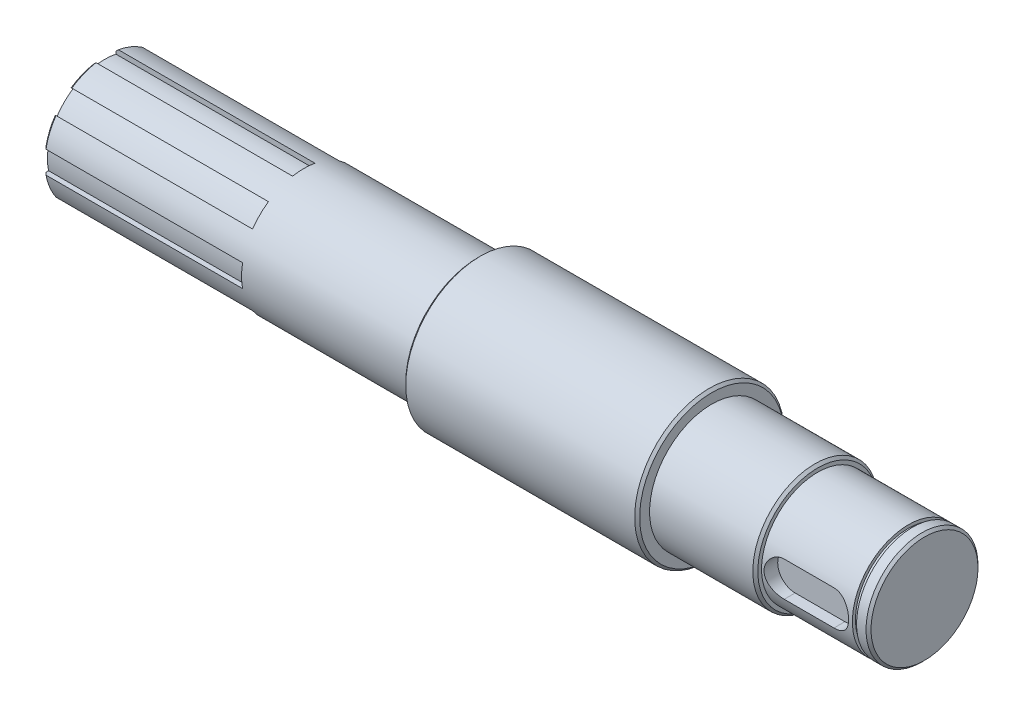
SolidWorks part; units mm, degrees
ref_plane "前视基准面" through (0, 0, 0) normal (0, 0, 1) x (1, 0, 0)
ref_plane "上视基准面" through (0, 0, 0) normal (0, 1, 0) x (1, 0, 0)
ref_plane "右视基准面" through (0, 0, 0) normal (1, 0, 0) x (0, 0, -1)
sketch "草图1" plane through (0, 0, 0) normal (0, 0, 1) x (1, 0, 0)
  line L0 (0, 0) -> (319.6501, 0) construction
  line L1 (0, 0) -> (0, 130.0325) construction
  line L2 (0, 0) -> (0, 25)
  line L3 (0, 25) -> (150, 25)
  line L4 (286.5, 25) -> (286.5, 22.5)
  line L5 (286.5, 22.5) -> (329.5, 22.5)
  line L6 (329.5, 22.5) -> (329.5, 0)
  line L7 (329.5, 0) -> (0, 0)
  line L8 (150, 25) -> (150, 30)
  line L9 (150, 30) -> (244, 30)
  line L10 (244, 30) -> (244, 25)
  line L11 (244, 25) -> (286.5, 25)
  dimension "D1" = 50
  dimension "D2" = 42.5
  dimension "D3" = 45
  dimension "D4" = 43
  dimension "D5" = 60
  dimension "D6" = 94
  dimension "D7" = 150
revolve "旋转1" add sketch "草图1" angle 360 about L7
chamfer "倒角1" distance 1 angle 45 4 edges at (329.5, 0, -22.5) (286.5, 0, -25) (244, 0, -30) (150, 0, -30)
ref_plane "基准面1" through (323, 0, 0) normal (1, 0, 0) x (0, 0, -1)
sketch "草图2" plane through (323, 0, 0) normal (1, 0, 0) x (0, 0, -1)
  circle A0 centre (0, 0) radius 21.25
  circle A1 centre (0, 0) radius 22.5
  dimension "D1" = 45
  dimension "D2" = 42.5
extrude "切除-拉伸1" cut sketch "草图2" along normal blind 1.7
ref_plane "基准面2" through (0, 0, 22.5) normal (0, 0, 1) x (1, 0, 0)
sketch "草图3" plane through (0, 0, 22.5) normal (0, 0, 1) x (1, 0, 0)
  line L0 (0, 0) -> (272.7051, 0) construction
  line L1 (294.5, 0) -> (314.5, 0) construction
  line L2 (294.5, 7) -> (314.5, 7)
  line L3 (294.5, -7) -> (314.5, -7)
  line L5 (329.5, -21.5) -> (329.5, 21.5) construction
  arc A0 (294.5, 7) -> (294.5, -7) centre (294.5, 0) ccw
  arc A1 (314.5, -7) -> (314.5, 7) centre (314.5, 0) ccw
  point P5 (304.5, 0)
  point P11 (321.5, 0)
  dimension "D2" = 20
  dimension "D1" = 14
  dimension "D3" = 8
extrude "切除-拉伸2" cut sketch "草图3" against normal blind 5.5
sketch "草图4" plane through (0, 0, 0) normal (-1, 0, 0) x (0, 0, 1)
  line L0 (0, 0) -> (0, 33.8685) construction
  line L1 (0, 0) -> (38.9741, 0) construction
  line L2 (-4.5, 24.5917) -> (-4.5, 22.5555)
  line L3 (4.5, 24.5917) -> (4.5, 22.5555)
  line L4 (20.5709, 14.207) -> (19.1311, 12.7672)
  line L5 (14.207, 20.5709) -> (12.7672, 19.1311)
  line L6 (24.5917, -4.5) -> (22.5555, -4.5)
  line L7 (24.5917, 4.5) -> (22.5555, 4.5)
  line L8 (14.207, -20.5709) -> (12.7672, -19.1311)
  line L9 (20.5709, -14.207) -> (19.1311, -12.7672)
  line L10 (-4.5, -24.5917) -> (-4.5, -22.5555)
  line L11 (4.5, -24.5917) -> (4.5, -22.5555)
  line L12 (-20.5709, -14.207) -> (-19.1311, -12.7672)
  line L13 (-14.207, -20.5709) -> (-12.7672, -19.1311)
  line L14 (-24.5917, 4.5) -> (-22.5555, 4.5)
  line L15 (-24.5917, -4.5) -> (-22.5555, -4.5)
  line L16 (-14.207, 20.5709) -> (-12.7672, 19.1311)
  line L17 (-20.5709, 14.207) -> (-19.1311, 12.7672)
  arc A0 (-12.7672, 19.1311) -> (-19.1311, 12.7672) centre (0, 0) ccw
  arc A1 (-14.207, 20.5709) -> (-20.5709, 14.207) centre (0, 0) ccw
  arc A2 (4.5, 22.5555) -> (-4.5, 22.5555) centre (0, 0) ccw
  arc A3 (4.5, 24.5917) -> (-4.5, 24.5917) centre (0, 0) ccw
  arc A4 (19.1311, 12.7672) -> (12.7672, 19.1311) centre (0, 0) ccw
  arc A5 (20.5709, 14.207) -> (14.207, 20.5709) centre (0, 0) ccw
  arc A6 (22.5555, -4.5) -> (22.5555, 4.5) centre (0, 0) ccw
  arc A7 (24.5917, -4.5) -> (24.5917, 4.5) centre (0, 0) ccw
  arc A8 (12.7672, -19.1311) -> (19.1311, -12.7672) centre (0, 0) ccw
  arc A9 (14.207, -20.5709) -> (20.5709, -14.207) centre (0, 0) ccw
  arc A10 (-4.5, -22.5555) -> (4.5, -22.5555) centre (0, 0) ccw
  arc A11 (-4.5, -24.5917) -> (4.5, -24.5917) centre (0, 0) ccw
  arc A12 (-19.1311, -12.7672) -> (-12.7672, -19.1311) centre (0, 0) ccw
  arc A13 (-20.5709, -14.207) -> (-14.207, -20.5709) centre (0, 0) ccw
  arc A14 (-22.5555, 4.5) -> (-22.5555, -4.5) centre (0, 0) ccw
  arc A15 (-24.5917, 4.5) -> (-24.5917, -4.5) centre (0, 0) ccw
  point P41 (0, 0)
  dimension "D1" = 46
  dimension "D2" = 50
  dimension "D3" = 9
  dimension "D4" = 8
extrude "切除-拉伸3" cut sketch "草图4" against normal blind 80
chamfer "倒角2" distance 1 angle 45 8 edges at (0, 23.097, -9.5671) (0, 9.5671, -23.097) (0, -9.5671, -23.097) (0, -23.097, -9.5671) (0, -23.097, 9.5671) (0, -9.5671, 23.097) (0, 9.5671, 23.097) (0, 23.097, 9.5671)
